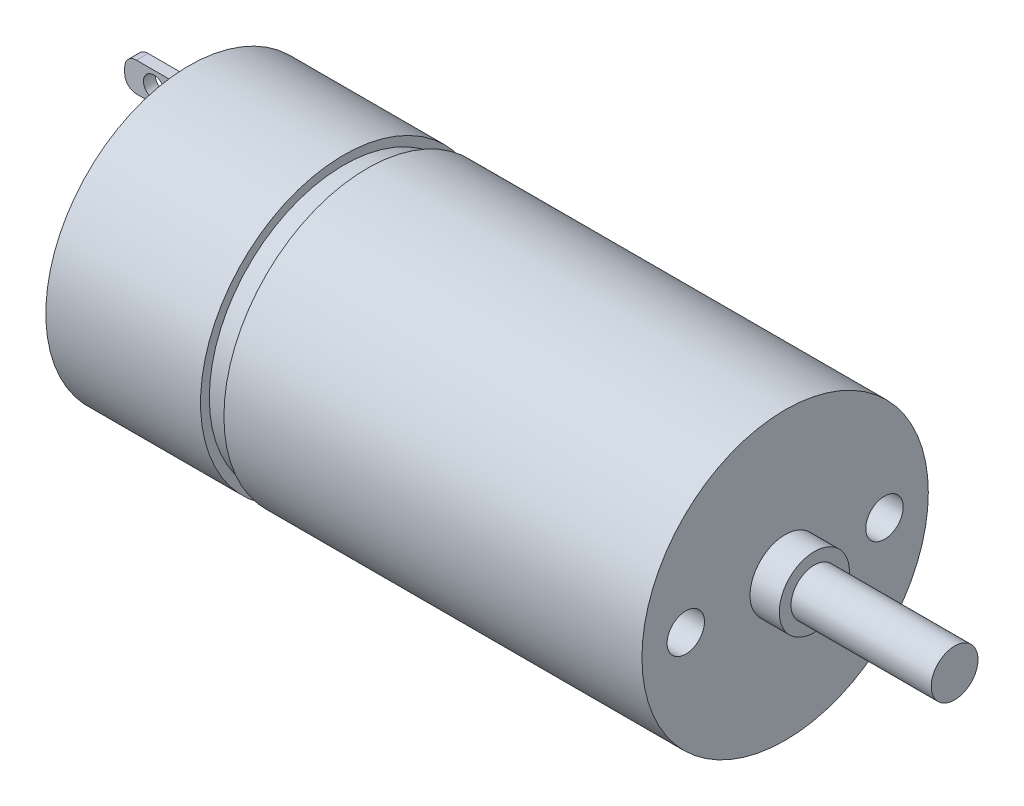
SolidWorks part; units mm, degrees
ref_plane "Front Plane" through (0, 0, 0) normal (0, 0, 1) x (1, 0, 0)
ref_plane "Top Plane" through (0, 0, 0) normal (0, 1, 0) x (1, 0, 0)
ref_plane "Right Plane" through (0, 0, 0) normal (1, 0, 0) x (0, 0, -1)
sketch "Sketch4" plane through (0, 0, 0) normal (1, 0, 0) x (0, 0, -1)
  circle A0 centre (0, 0) radius 12.25
  dimension "D1" = 24.5
extrude "Boss-Extrude1" add sketch "Sketch4" along normal blind 51
sketch "Sketch5" plane through (0, 0, 0) normal (0, 0, 1) x (1, 0, 0)
  line L0 (0, 12.25) -> (0, -12.25) construction
  line L1 (-5, 10.9036) -> (0, 10.9036)
  line L2 (-5, 10.9036) -> (-5, 8.4036)
  line L3 (-5, 8.4036) -> (0, 8.4036)
  line L4 (0, 10.9036) -> (0, 8.4036)
  line L5 (-5, 10.9036) -> (0, 8.4036) construction
  line L6 (-5, 8.4036) -> (0, 10.9036) construction
  line L7 (-7.0132, 0) -> (60.6917, 0) construction
  line L8 (-5, -8.4036) -> (0, -10.9036) construction
  line L9 (-5, -10.9036) -> (0, -8.4036) construction
  line L10 (0, -10.9036) -> (0, -8.4036)
  line L11 (-5, -8.4036) -> (0, -8.4036)
  line L12 (-5, -10.9036) -> (-5, -8.4036)
  line L13 (-5, -10.9036) -> (0, -10.9036)
  circle A0 centre (-2.5, 9.6536) radius 0.9
  circle A1 centre (-2.5, -9.6536) radius 0.9
  point P0 (-2.5, 9.6536)
  dimension "D3" = 1.8
  dimension "D1" = 5
  dimension "D2" = 2.5
extrude "Boss-Extrude2" add sketch "Sketch5" along normal mid plane 1
fillet "Fillet1" radius 1 4 edges at (-5, -8.4036, 0) (-5, -10.9036, 0) (-5, 8.4036, 0) (-5, 10.9036, 0)
sketch "Sketch6" plane through (51, 0, 0) normal (1, 0, 0) x (0, 0, -1)
  circle A1 centre (0, 0) radius 3
  dimension "D2" = 6
extrude "Boss-Extrude3" add sketch "Sketch6" along normal blind 2.5
sketch "Sketch7" plane through (53.5, 0, 0) normal (1, 0, 0) x (0, 0, -1)
  circle A0 centre (0, 0) radius 2
  dimension "D1" = 4
extrude "Boss-Extrude4" add sketch "Sketch7" along normal blind 12
sketch "Sketch8" plane through (0, 0, 0) normal (0, 0, 1) x (1, 0, 0)
  line L0 (51, 12.25) -> (0, 12.25) construction
  line L1 (13.2357, 15) -> (15.2357, 15)
  line L2 (13.2357, 15) -> (13.2357, 11.5)
  line L3 (13.2357, 11.5) -> (15.2357, 11.5)
  line L4 (15.2357, 15) -> (15.2357, 11.5)
  line L5 (13.2357, 15) -> (15.2357, 11.5) construction
  line L6 (13.2357, 11.5) -> (15.2357, 15) construction
  line L7 (-4.3663, 0) -> (69.6625, 0) construction
  point P0 (14.2357, 13.25)
  dimension "D1" = 3.5
  dimension "D2" = 2
  dimension "D3" = 1
revolve "Cut-Revolve1" cut sketch "Sketch8" angle 360 about L7
sketch "Sketch9" plane through (51, 0, 0) normal (1, 0, 0) x (0, 0, -1)
  line L0 (0, 0) -> (8.5, 0) construction
  line L1 (8.5, 0) -> (-8.5, 0) construction
  circle A0 centre (-8.5, 0) radius 1.6
  circle A1 centre (8.5, 0) radius 1.6
  dimension "D1" = 8.5
  dimension "D2" = 17
extrude "Cut-Extrude1" cut sketch "Sketch9" against normal blind 5
